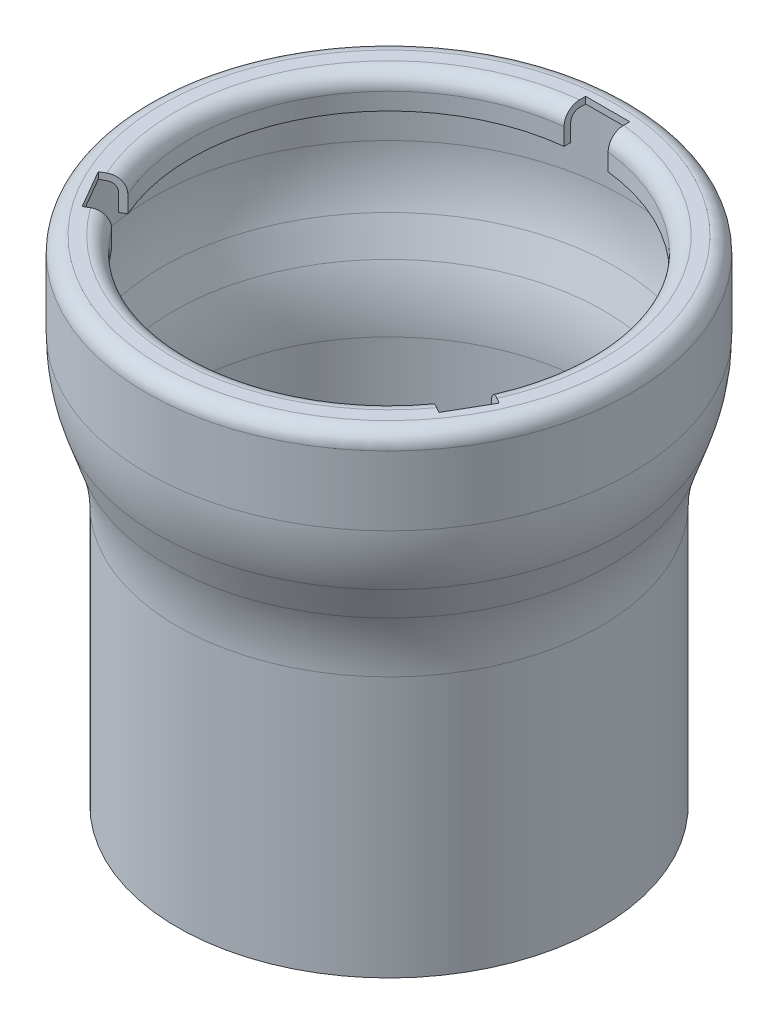
SolidWorks part; units mm, degrees
material "Q235"
ref_plane "Front Plane" through (0, 0, 0) normal (0, 0, 1) x (1, 0, 0)
ref_plane "Top Plane" through (0, 0, 0) normal (0, 1, 0) x (1, 0, 0)
ref_plane "Right Plane" through (0, 0, 0) normal (1, 0, 0) x (0, 0, -1)
sketch "Sketch1" plane through (0, 0, 0) normal (0, 0, 1) x (1, 0, 0)
  line L0 (48, 0) -> (48, 59.1567)
  line L1 (50.2145, 72.2812) -> (52.7855, 79.6834)
  line L2 (55, 92.8079) -> (55, 108.5)
  line L3 (51.5, 112) -> (48.5, 112)
  line L4 (45, 108.5) -> (45, 104.6154)
  line L5 (46.5, 0) -> (46.5, 59.1567)
  line L6 (48.7975, 72.7734) -> (51.3686, 80.1756)
  line L7 (53.5, 92.8079) -> (53.5, 108.5)
  line L8 (51.5, 110.5) -> (48.5, 110.5)
  line L9 (46.5, 108.5) -> (46.5, 104.6154)
  line L10 (45, 104.6154) -> (46.5, 104.6154)
  line L11 (46.5, 0) -> (48, 0)
  line L12 (0, 0) -> (0, 44.8472) construction
  arc A0 (55, 108.5) -> (51.5, 112) centre (51.5, 108.5) ccw
  arc A1 (48.5, 112) -> (45, 108.5) centre (48.5, 108.5) ccw
  arc A2 (48, 59.1567) -> (50.2145, 72.2812) centre (88, 59.1567) cw
  arc A3 (52.7855, 79.6834) -> (55, 92.8079) centre (15, 92.8079) ccw
  arc A4 (46.5, 59.1567) -> (48.7975, 72.7734) centre (88, 59.1567) cw
  arc A5 (51.3686, 80.1756) -> (53.5, 92.8079) centre (15, 92.8079) ccw
  arc A6 (53.5, 108.5) -> (51.5, 110.5) centre (51.5, 108.5) ccw
  arc A7 (48.5, 110.5) -> (46.5, 108.5) centre (48.5, 108.5) ccw
  dimension "D5" = 3.5
  dimension "D6" = 40
  dimension "D1" = 48
  dimension "D2" = 55
  dimension "D3" = 112
  dimension "D4" = 10
  dimension "D7" = 1.5
revolve "Revolve1" add sketch "Sketch1" angle 360 about L12
sketch "Sketch2" plane through (0, 112, 0) normal (0, 1, 0) x (1, 0, 0)
  line L1 (-5, 29.802) -> (5, 29.802)
  line L2 (-5, 29.802) -> (-5, 49.6255)
  line L3 (-5, 49.6255) -> (5, 49.6255)
  line L4 (5, 29.802) -> (5, 49.6255)
  line L5 (0, 49.6255) -> (0, 29.802) construction
  line L6 (-5, 39.7138) -> (5, 39.7138) construction
  point P0 (0, 39.7138)
  dimension "D1" = 10
extrude "Cut-Extrude1" cut sketch "Sketch2" against normal blind 10
pattern_circular "CirPattern1" count 3 over 360 about axis through (0, 0, 0) along (0, 1, 0) of "Cut-Extrude1"
